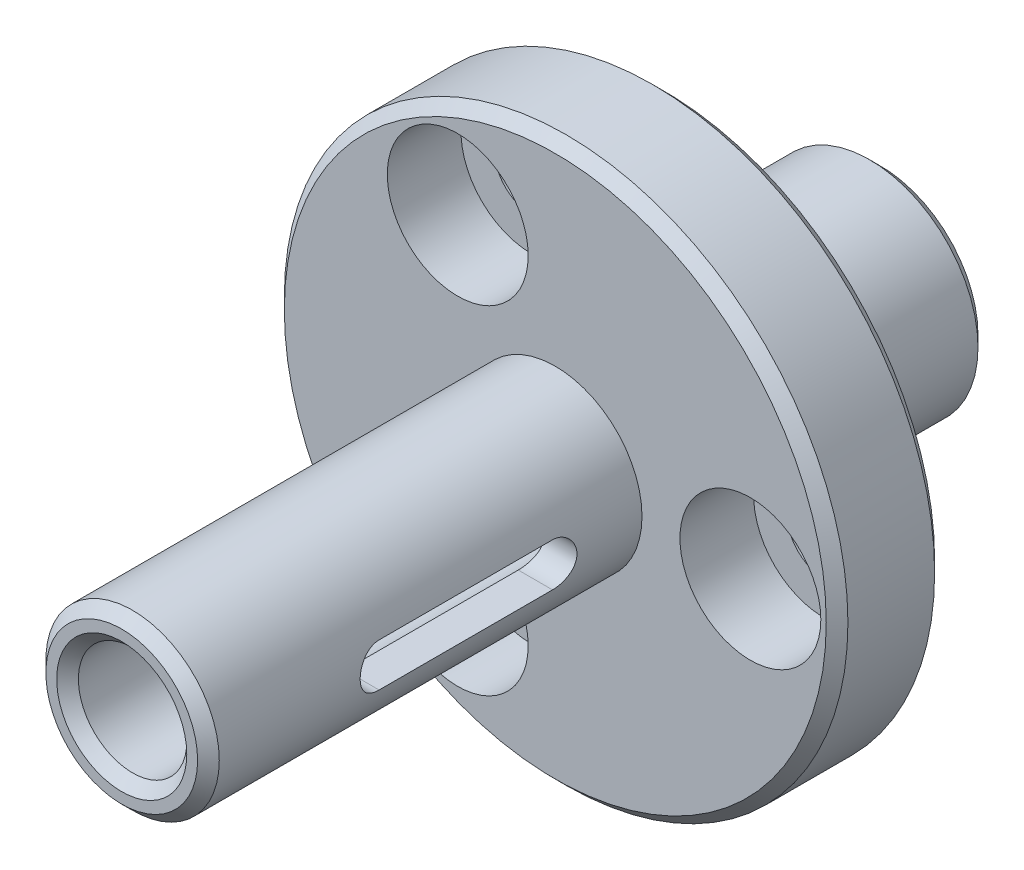
SolidWorks part; units mm, degrees
material "S45C"
ref_plane "Front Plane" through (0, 0, 0) normal (0, 0, 1) x (1, 0, 0)
ref_plane "Top Plane" through (0, 0, 0) normal (0, 1, 0) x (1, 0, 0)
ref_plane "Right Plane" through (0, 0, 0) normal (1, 0, 0) x (0, 0, -1)
sketch "Sketch1" plane through (0, 0, 0) normal (0, 0, 1) x (1, 0, 0)
  circle A0 centre (0, 0) radius 5
  dimension "D1" = 10
extrude "Boss-Extrude1" add sketch "Sketch1" along normal blind 10
sketch "Sketch2" plane through (0, 0, 10) normal (0, 0, 1) x (1, 0, 0)
  circle A0 centre (0, 0) radius 13
  dimension "D1" = 26
extrude "Boss-Extrude2" add sketch "Sketch2" along normal blind 5
sketch "Sketch3" plane through (0, 0, 15) normal (0, 0, 1) x (1, 0, 0)
  circle A0 centre (0, 0) radius 4
  dimension "D1" = 8
extrude "Boss-Extrude3" add sketch "Sketch3" along normal blind 20
sketch "Sketch4" plane through (0, 0, 35) normal (0, 0, 1) x (1, 0, 0)
  circle A0 centre (0, 0) radius 2.5
  dimension "D1" = 5
extrude "Cut-Extrude1" cut sketch "Sketch4" against normal blind 30
hole_wizard "CBORE for M3 Hex Socket Head Cap Screw1" positions "Sketch6" profile "Sketch5" counterbore size "M3" standard "Iso" end condition through all
sketch "Sketch6" plane through (0, 0, 15) normal (0, 0, 1) x (1, 0, 0)
  line L0 (0, 0) -> (13, 0) construction
  circle A0 centre (0, 0) radius 13 construction
  point P0 (9, 0)
  dimension "D1" = 9
sketch "Sketch5" plane through (9, 0, 15) normal (1, 0, 0) x (0, -1, 0)
  line L0 (0, 0) -> (0, 15)
  line L1 (0, 15) -> (1.7, 15)
  line L3 (1.7, 15) -> (1.7, 3.4)
  line L4 (1.7, 3.4) -> (3.25, 3.4)
  line L5 (3.25, 3.4) -> (3.25, 0)
  line L7 (3.25, 0) -> (0, 0)
  line L11 (0, -6.35) -> (0, 107.95) construction
  dimension "通孔孔直径" = 3.4
  dimension "通孔孔深度" = 15
  dimension "柱形沉头孔直径" = 6.5
  dimension "柱形沉头孔深度" = 3.4
pattern_circular "CirPattern1" count 3 over 360 about axis through (0, 0, 0) along (0, 0, 1) of "CBORE for M3 Hex Socket Head Cap Screw1"
ref_plane "Plane1" through (4, 0, 0) normal (1, 0, 0) x (0, 0, -1)
sketch "Sketch7" plane through (4, 0, 0) normal (1, 0, 0) x (0, 0, -1)
  line L0 (-35, 0) -> (-15, 0) construction
  line L1 (-35, 4) -> (-35, -4) construction
  line L2 (-15, 13) -> (-15, -13) construction
  line L3 (-27, 0) -> (-19, 0) construction
  line L4 (-27, 1) -> (-19, 1)
  line L5 (-27, -1) -> (-19, -1)
  arc A0 (-27, 1) -> (-27, -1) centre (-27, 0) ccw
  arc A1 (-19, -1) -> (-19, 1) centre (-19, 0) ccw
  point P8 (-23, 0)
  dimension "D1" = 8
  dimension "D2" = 8
  dimension "D3" = 2
extrude "Cut-Extrude2" cut sketch "Sketch7" against normal through all
chamfer "Chamfer1" distance 0.5 angle 45 5 edges at (2.5, 0, 35) (4, 0, 35) (13, 0, 15) (13, 0, 10) (5, 0, 0)
